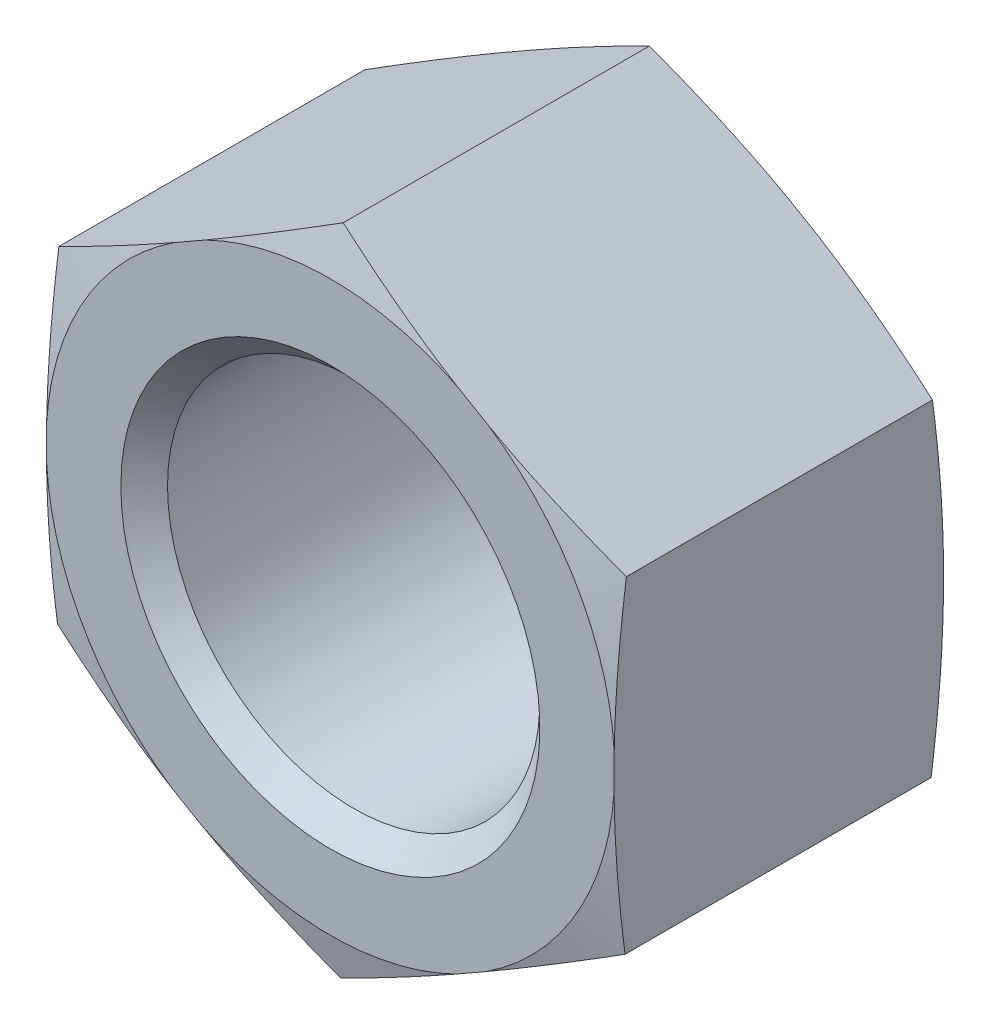
SolidWorks part; units mm, degrees
material "SAE2"
ref_plane "Plane1" through (0, 0, 0) normal (0, 0, 1) x (1, 0, 0)
ref_plane "Plane2" through (0, 0, 0) normal (0, 1, 0) x (1, 0, 0)
ref_plane "Plane3" through (0, 0, 0) normal (1, 0, 0) x (0, 0, -1)
sketch "Dimension sketch" plane through (0, 0, 0) normal (0, 0, 1) x (1, 0, 0)
  line L0 (0, 0) -> (-1.4751, 0)
  line L1 (-1.4751, 0) -> (37.4249, 0)
  line L2 (37.4249, 0) -> (88.5249, 0)
  line L3 (-34.2857, 0) -> (0, 0)
  point P3 (36, 0)
  point P4 (1.5, 0)
  point P5 (60.79, 0)
  point P6 (31, 0)
  point P7 (6.4, 0)
  point P8 (55, 0)
  dimension "D1" = 34.2857
  dimension "D" = 36
  dimension "P" = 1.5
  dimension "e" = 60.79
  dimension "m" = 31
  dimension "mw" = 6.4
  dimension "s" = 55
  dimension "da" = 38.9
  dimension "dw" = 51.1
sketch "Sketch1" plane through (0, 0, 0) normal (0, 0, 1) x (1, 0, 0)
  line L0 (-26.8088, 0) -> (37.1748, 0) construction
  line L1 (0, 25.0215) -> (0, -25.0215) construction
  line L3 (0.1274, 32.3847) -> (-27.9823, 16.3027)
  line L4 (-27.9823, 16.3027) -> (-28.1097, -16.0821)
  line L5 (-28.1097, -16.0821) -> (-0.1274, -32.3847)
  line L6 (-0.1274, -32.3847) -> (27.9823, -16.3027)
  line L7 (27.9823, -16.3027) -> (28.1097, 16.0821)
  line L8 (28.1097, 16.0821) -> (0.1274, 32.3847)
  circle A0 centre (0, 0) radius 28.0462 construction
  circle A1 centre (0, 0) radius 18.4
  dimension "D" = 36.8
  dimension "e" = 64.77
extrude "Base-Extrude" add sketch "Sketch1" along normal blind 32.5437
cosmetic thread "Cosmetic Thread1" parameters "D2"=36
sketch "Sketch2" plane through (0, 0, 0) normal (0, 0, -1) x (-1, 0, 0)
  circle A0 centre (0, 0) radius 28.1
  circle A1 centre (0, 0) radius 18.4 construction
  dimension "s" = 56.2
extrude "Cut-Extrude1" cut sketch "Sketch2" against normal through all draft 75 flip side to cut
sketch "Sketch3" plane through (0, 0, 32.5437) normal (0, 0, 1) x (1, 0, 0)
  circle A0 centre (0, 0) radius 28.1
  dimension "D1" = 56.2
extrude "Cut-Extrude2" cut sketch "Sketch3" against normal through all draft 75 flip side to cut
chamfer "Chamfer1" distance 2.3071 angle 45 2 edges at (18.4, 0, 0) (18.4, 0, 32.5437)
